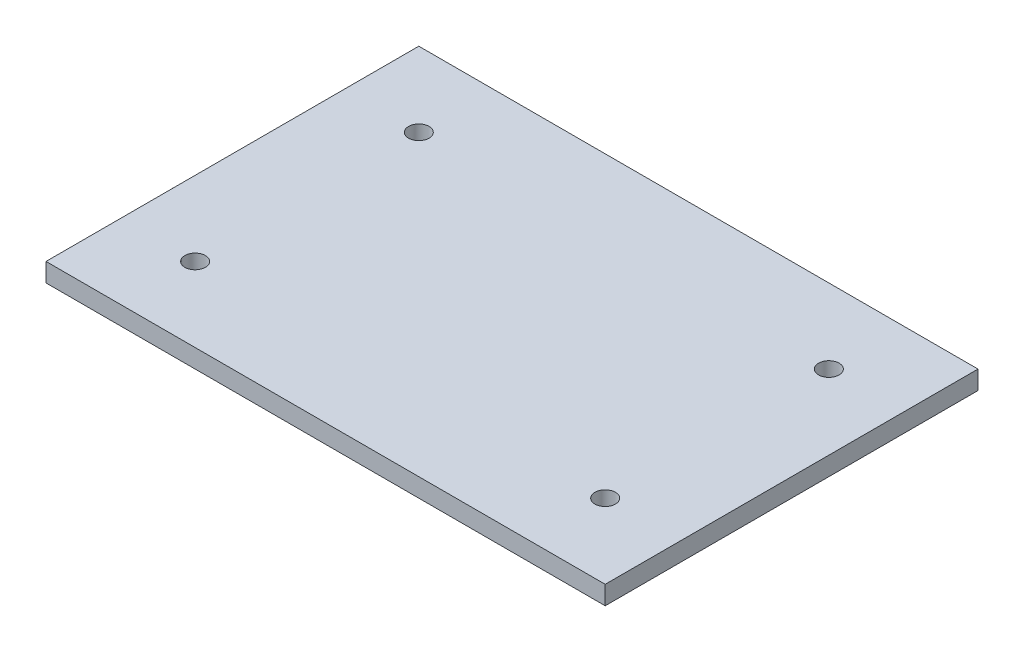
SolidWorks part; units mm, degrees
ref_plane "Front Plane" through (0, 0, 0) normal (0, 0, 1) x (1, 0, 0)
ref_plane "Top Plane" through (0, 0, 0) normal (0, 1, 0) x (1, 0, 0)
ref_plane "Right Plane" through (0, 0, 0) normal (1, 0, 0) x (0, 0, -1)
other "Configuration Table"
sketch "Sketch1" plane through (0, 0, 0) normal (0, 1, 0) x (1, 0, 0)
  line L1 (-300, -200) -> (300, -200)
  line L2 (-300, -200) -> (-300, 200)
  line L3 (-300, 200) -> (300, 200)
  line L4 (300, -200) -> (300, 200)
  line L5 (-300, -200) -> (300, 200) construction
  line L6 (-300, 200) -> (300, -200) construction
  point P0 (0, 0)
  dimension "D1" = 600
  dimension "D2" = 400
extrude "Boss-Extrude1" add sketch "Sketch1" along normal blind 20
sketch "Sketch2" plane through (0, 20, 0) normal (0, 1, 0) x (1, 0, 0)
  line L0 (0, 200) -> (0, -200) construction
  line L1 (300, 200) -> (-300, 200) construction
  line L2 (-300, -200) -> (300, -200) construction
  line L3 (-300, 0) -> (300, 0) construction
  line L4 (-300, 200) -> (-300, -200) construction
  line L5 (300, -200) -> (300, 200) construction
  circle A0 centre (-220, 120) radius 11
  circle A3 centre (220, 120) radius 11
  circle A4 centre (220, -120) radius 11
  circle A5 centre (-220, -120) radius 11
  dimension "D1" = 22
  dimension "D2" = 120
  dimension "D3" = 220
extrude "Cut-Extrude1" cut sketch "Sketch2" against normal blind 20
